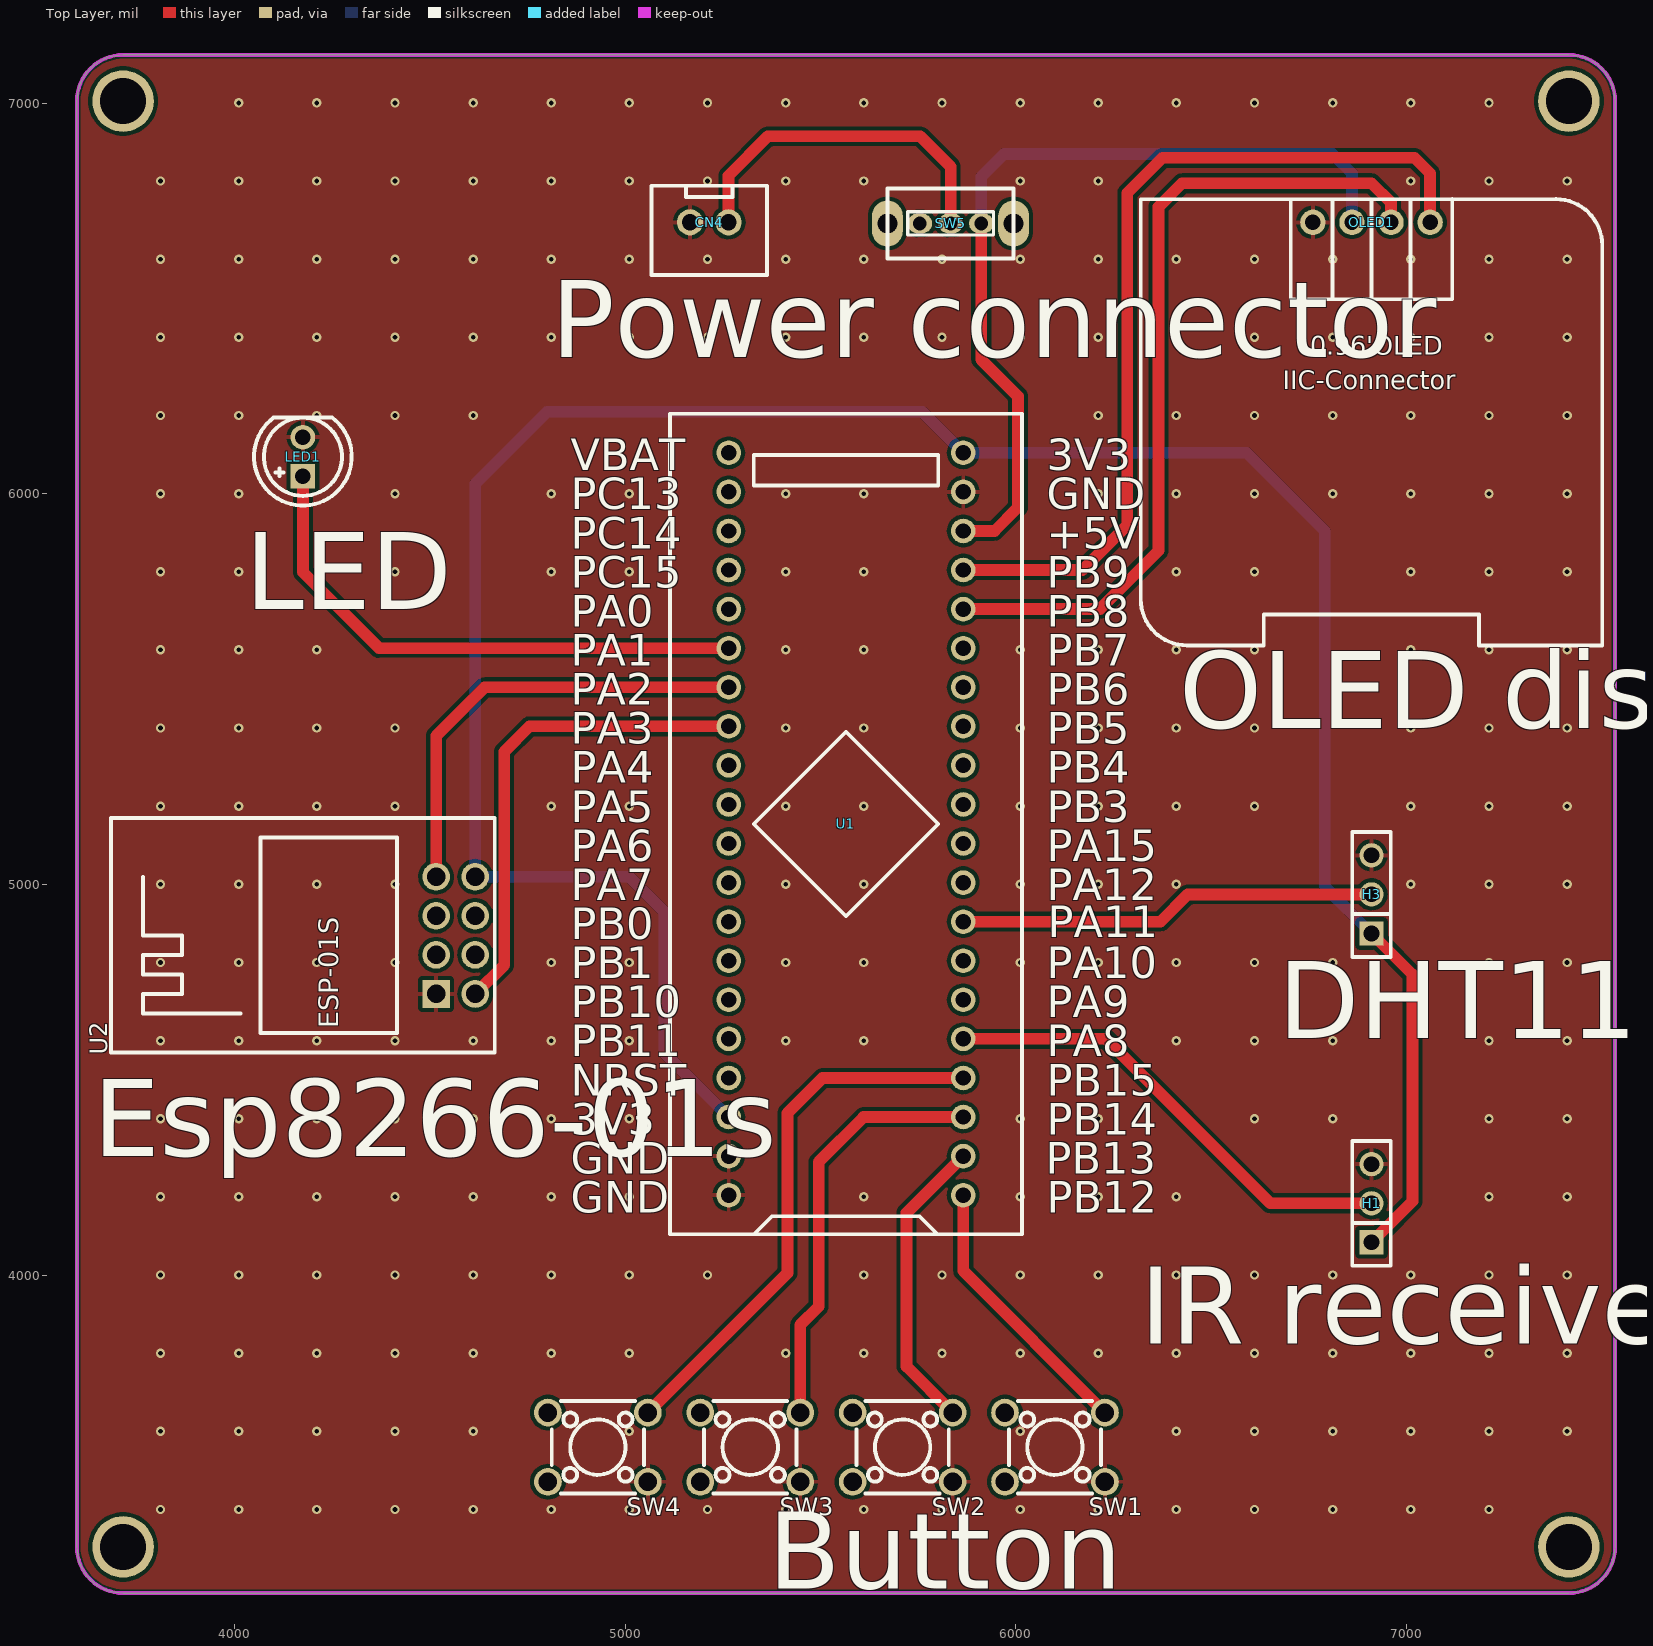
[diagram p0: Top Layer view]
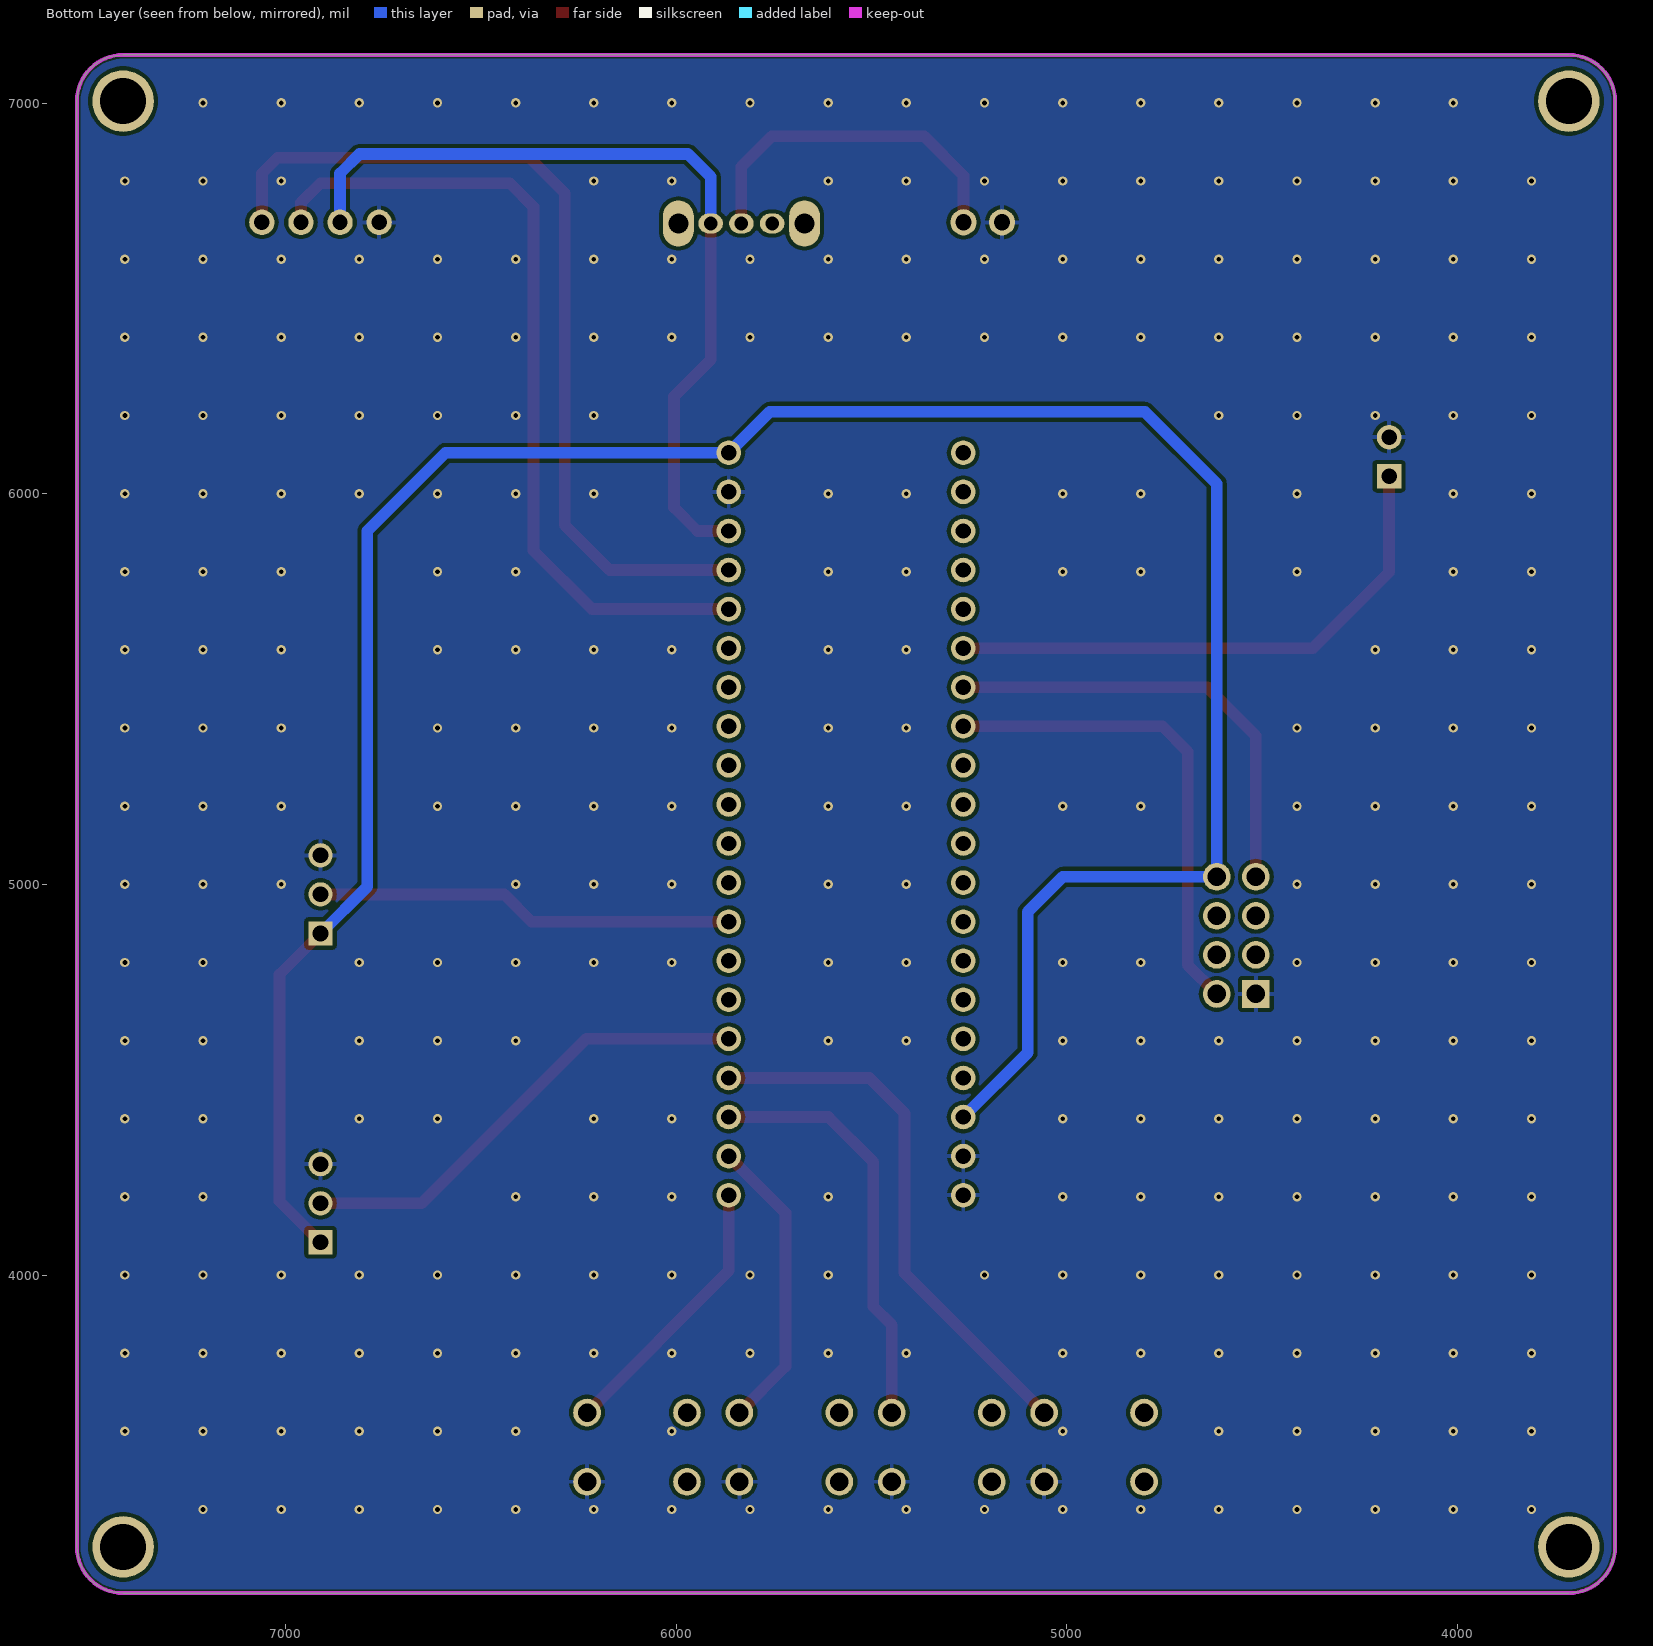
[diagram p1: Bottom Layer view, seen from below]
# Altium PCB MISC49868.pcbdoc
Units mil, origin at the board's own origin, x right, y up, seen from the top; angles counter-clockwise.
Board outline 3937.01 x 3937.01 mil, 2 copper layers (Top Layer, Bottom Layer), stack 62.206 mil thick; 12 components, 38 nets, 87 pads, 282 vias.

## Layer stack, top to bottom
Top Solder Mask Layer: solder mask 0.394, Dk 3.3
Top Layer: signal copper 1.379
Dielectric1: surface 59.449, FR4, Dk 4.5
Bottom Layer: signal copper 1.378
Bottom Solder Mask Layer: solder mask 0.394, Dk 3.3

## Board outline
3714.61,7123.5 ccw(c3714.61,7005.39) 3596.5,7005.39 3596.5,3304.61 ccw(c3714.61,3304.61) 3714.61,3186.5 7415.39,3186.5 ccw(c7415.39,3304.61) 7533.5,3304.61 7533.5,7005.39 ccw(c7415.39,7005.39) 7415.39,7123.5 3714.61,7123.5

## Design rules (kind name [scope] priority, off if disabled: settings)
BoardOutlineClearance copperThickness2oz_1 [All] p2 off: genericclearance=7.99 ignorepadtopadclearanceinfootprint=FALSE except(0: Arc-SplitContinuation Track-SplitContinuation SMDPad-SplitContinuation THPad-SplitContinuation Via-SplitContinuation Fill-SplitContinuation Region-SplitContinuation Poly-SplitContinuation Text-SplitContinuation Hole-SplitContinuation; 5.98: Arc-CutoutEdge Track-CutoutEdge SMDPad-CutoutEdge THPad-CutoutEdge Via-CutoutEdge Text-CutoutEdge; 6.9: Hole-OutlineEdge Hole-CutoutEdge; 10: Poly-OutlineEdge Poly-CutoutEdge; 11.81: Arc-OutlineEdge Track-OutlineEdge SMDPad-OutlineEdge THPad-OutlineEdge Via-OutlineEdge Fill-OutlineEdge Region-OutlineEdge Text-OutlineEdge Fill-CutoutEdge Region-CutoutEdge)
BoardOutlineClearance Plane_innerPlane_1 [All] p4 off: genericclearance=4.02 ignorepadtopadclearanceinfootprint=FALSE except(0: Arc-SplitContinuation Track-SplitContinuation SMDPad-SplitContinuation THPad-SplitContinuation Via-SplitContinuation Fill-SplitContinuation Region-SplitContinuation Poly-SplitContinuation Text-SplitContinuation Hole-SplitContinuation; 5.98: Arc-CutoutEdge Track-CutoutEdge SMDPad-CutoutEdge THPad-CutoutEdge Via-CutoutEdge Text-CutoutEdge; 6.9: Hole-OutlineEdge Hole-CutoutEdge; 10: Poly-OutlineEdge Poly-CutoutEdge; 11.81: Arc-OutlineEdge Track-OutlineEdge SMDPad-OutlineEdge THPad-OutlineEdge Via-OutlineEdge Fill-OutlineEdge Region-OutlineEdge Text-OutlineEdge Fill-CutoutEdge Region-CutoutEdge)
BoardOutlineClearance Copper_copperRegion_1 [All] p6 off: genericclearance=4.02 ignorepadtopadclearanceinfootprint=FALSE except(0: Arc-SplitContinuation Track-SplitContinuation SMDPad-SplitContinuation THPad-SplitContinuation Via-SplitContinuation Fill-SplitContinuation Region-SplitContinuation Poly-SplitContinuation Text-SplitContinuation Hole-SplitContinuation; 5.98: Arc-CutoutEdge Track-CutoutEdge SMDPad-CutoutEdge THPad-CutoutEdge Via-CutoutEdge Text-CutoutEdge; 6.9: Hole-OutlineEdge Hole-CutoutEdge; 10: Poly-OutlineEdge Poly-CutoutEdge; 11.81: Arc-OutlineEdge Track-OutlineEdge SMDPad-OutlineEdge THPad-OutlineEdge Via-OutlineEdge Fill-OutlineEdge Region-OutlineEdge Text-OutlineEdge Fill-CutoutEdge Region-CutoutEdge)
BoardOutlineClearance Copper_copperRegion_copperThickness1oz_1 [All] p8 off: genericclearance=4.02 ignorepadtopadclearanceinfootprint=FALSE except(0: Arc-SplitContinuation Track-SplitContinuation SMDPad-SplitContinuation THPad-SplitContinuation Via-SplitContinuation Fill-SplitContinuation Region-SplitContinuation Poly-SplitContinuation Text-SplitContinuation Hole-SplitContinuation; 5.98: Arc-CutoutEdge Track-CutoutEdge SMDPad-CutoutEdge THPad-CutoutEdge Via-CutoutEdge Text-CutoutEdge; 6.9: Hole-OutlineEdge Hole-CutoutEdge; 10: Poly-OutlineEdge Poly-CutoutEdge; 11.81: Arc-OutlineEdge Track-OutlineEdge SMDPad-OutlineEdge THPad-OutlineEdge Via-OutlineEdge Fill-OutlineEdge Region-OutlineEdge Text-OutlineEdge Fill-CutoutEdge Region-CutoutEdge)
BoardOutlineClearance Copper_copperRegion_Copper_copperRegion_1 [All] p10 off: genericclearance=4.02 ignorepadtopadclearanceinfootprint=FALSE except(0: Arc-SplitContinuation Track-SplitContinuation SMDPad-SplitContinuation THPad-SplitContinuation Via-SplitContinuation Fill-SplitContinuation Region-SplitContinuation Poly-SplitContinuation Text-SplitContinuation Hole-SplitContinuation; 5.98: Arc-CutoutEdge Track-CutoutEdge SMDPad-CutoutEdge THPad-CutoutEdge Via-CutoutEdge Text-CutoutEdge; 6.9: Hole-OutlineEdge Hole-CutoutEdge; 10: Poly-OutlineEdge Poly-CutoutEdge; 11.81: Arc-OutlineEdge Track-OutlineEdge SMDPad-OutlineEdge THPad-OutlineEdge Via-OutlineEdge Fill-OutlineEdge Region-OutlineEdge Text-OutlineEdge Fill-CutoutEdge Region-CutoutEdge)
BoardOutlineClearance copperThickness1oz_1 [All] p12: genericclearance=4.02 ignorepadtopadclearanceinfootprint=FALSE except(0: Arc-SplitContinuation Track-SplitContinuation SMDPad-SplitContinuation THPad-SplitContinuation Via-SplitContinuation Fill-SplitContinuation Region-SplitContinuation Poly-SplitContinuation Text-SplitContinuation Hole-SplitContinuation; 5.98: Arc-CutoutEdge Track-CutoutEdge SMDPad-CutoutEdge THPad-CutoutEdge Via-CutoutEdge Text-CutoutEdge; 6.9: Hole-OutlineEdge Hole-CutoutEdge; 10: Poly-OutlineEdge Poly-CutoutEdge; 11.81: Arc-OutlineEdge Track-OutlineEdge SMDPad-OutlineEdge THPad-OutlineEdge Via-OutlineEdge Fill-OutlineEdge Region-OutlineEdge Text-OutlineEdge Fill-CutoutEdge Region-CutoutEdge)
Clearance copperThickness2oz [All] p1 off: gap=7.99 ignorepadtopadclearanceinfootprint=FALSE except(5.98: SMDPad-Track SMDPad-SMDPad THPad-Track SMDPad-THPad THPad-THPad Track-Via SMDPad-Via THPad-Via Via-Via Fill-SMDPad Region-SMDPad Fill-THPad Region-THPad Fill-Via Region-Via Fill-Fill Fill-Region Region-Region Arc-Track Arc-SMDPad Arc-THPad Arc-Via Fill-Arc Region-Arc Arc-Arc Text-Track SMDPad-Text Text-THPad Text-Via Fill-Text Region-Text Arc-Text Text-Text; 6.9: Hole-Track Hole-SMDPad Hole-THPad Hole-Via Fill-Hole Region-Hole Hole-Arc Hole-Text; 10: Poly-Track Poly-SMDPad Poly-THPad Poly-Via Poly-Fill Poly-Region Poly-Poly Poly-Arc Poly-Text Poly-Hole; 11.81: Fill-Track Region-Track)
Clearance Plane_innerPlane [All] p3 off: gap=4.02 ignorepadtopadclearanceinfootprint=FALSE except(5.98: SMDPad-Track SMDPad-SMDPad THPad-Track SMDPad-THPad THPad-THPad Track-Via SMDPad-Via THPad-Via Via-Via Fill-SMDPad Region-SMDPad Fill-THPad Region-THPad Fill-Via Region-Via Fill-Fill Fill-Region Region-Region Arc-Track Arc-SMDPad Arc-THPad Arc-Via Fill-Arc Region-Arc Arc-Arc Text-Track SMDPad-Text Text-THPad Text-Via Fill-Text Region-Text Arc-Text Text-Text; 6.9: Hole-Track Hole-SMDPad Hole-THPad Hole-Via Fill-Hole Region-Hole Hole-Arc Hole-Text; 10: Poly-Track Poly-SMDPad Poly-THPad Poly-Via Poly-Fill Poly-Region Poly-Poly Poly-Arc Poly-Text Poly-Hole; 11.81: Fill-Track Region-Track)
Clearance Copper_copperRegion [All] p5 off: gap=4.02 ignorepadtopadclearanceinfootprint=FALSE except(5.98: SMDPad-Track SMDPad-SMDPad THPad-Track SMDPad-THPad THPad-THPad Track-Via SMDPad-Via THPad-Via Via-Via Fill-SMDPad Region-SMDPad Fill-THPad Region-THPad Fill-Via Region-Via Fill-Fill Fill-Region Region-Region Arc-Track Arc-SMDPad Arc-THPad Arc-Via Fill-Arc Region-Arc Arc-Arc Text-Track SMDPad-Text Text-THPad Text-Via Fill-Text Region-Text Arc-Text Text-Text; 6.9: Hole-Track Hole-SMDPad Hole-THPad Hole-Via Fill-Hole Region-Hole Hole-Arc Hole-Text; 10: Poly-Track Poly-SMDPad Poly-THPad Poly-Via Poly-Fill Poly-Region Poly-Poly Poly-Arc Poly-Text Poly-Hole; 11.81: Fill-Track Region-Track)
Clearance Copper_copperRegion_copperThickness1oz [All] p7 off: gap=4.02 ignorepadtopadclearanceinfootprint=FALSE except(5.98: SMDPad-Track SMDPad-SMDPad THPad-Track SMDPad-THPad THPad-THPad Track-Via SMDPad-Via THPad-Via Via-Via Fill-SMDPad Region-SMDPad Fill-THPad Region-THPad Fill-Via Region-Via Fill-Fill Fill-Region Region-Region Arc-Track Arc-SMDPad Arc-THPad Arc-Via Fill-Arc Region-Arc Arc-Arc Text-Track SMDPad-Text Text-THPad Text-Via Fill-Text Region-Text Arc-Text Text-Text; 6.9: Hole-Track Hole-SMDPad Hole-THPad Hole-Via Fill-Hole Region-Hole Hole-Arc Hole-Text; 10: Poly-Track Poly-SMDPad Poly-THPad Poly-Via Poly-Fill Poly-Region Poly-Poly Poly-Arc Poly-Text Poly-Hole; 11.81: Fill-Track Region-Track)
Clearance Copper_copperRegion_Copper_copperRegion [All] p9 off: gap=4.02 ignorepadtopadclearanceinfootprint=FALSE except(5.98: SMDPad-Track SMDPad-SMDPad THPad-Track SMDPad-THPad THPad-THPad Track-Via SMDPad-Via THPad-Via Via-Via Fill-SMDPad Region-SMDPad Fill-THPad Region-THPad Fill-Via Region-Via Fill-Fill Fill-Region Region-Region Arc-Track Arc-SMDPad Arc-THPad Arc-Via Fill-Arc Region-Arc Arc-Arc Text-Track SMDPad-Text Text-THPad Text-Via Fill-Text Region-Text Arc-Text Text-Text; 6.9: Hole-Track Hole-SMDPad Hole-THPad Hole-Via Fill-Hole Region-Hole Hole-Arc Hole-Text; 10: Poly-Track Poly-SMDPad Poly-THPad Poly-Via Poly-Fill Poly-Region Poly-Poly Poly-Arc Poly-Text Poly-Hole; 11.81: Fill-Track Region-Track)
Clearance copperThickness1oz [All] p11: gap=4.02 ignorepadtopadclearanceinfootprint=FALSE except(5.98: SMDPad-Track SMDPad-SMDPad THPad-Track SMDPad-THPad THPad-THPad Track-Via SMDPad-Via THPad-Via Via-Via Fill-SMDPad Region-SMDPad Fill-THPad Region-THPad Fill-Via Region-Via Fill-Fill Fill-Region Region-Region Arc-Track Arc-SMDPad Arc-THPad Arc-Via Fill-Arc Region-Arc Arc-Arc Text-Track SMDPad-Text Text-THPad Text-Via Fill-Text Region-Text Arc-Text Text-Text; 6.9: Hole-Track Hole-SMDPad Hole-THPad Hole-Via Fill-Hole Region-Hole Hole-Arc Hole-Text; 10: Poly-Track Poly-SMDPad Poly-THPad Poly-Via Poly-Fill Poly-Region Poly-Poly Poly-Arc Poly-Text Poly-Hole; 11.81: Fill-Track Region-Track)
DiffPairsRouting differentialPair [All] p1: maxlimit=6 minlimit=6 mostfreqgap=6 toplayer_minwidth=5 toplayer_prefwidth=10 toplayer_maxwidth=100 toplayer_mingap=6 toplayer_prefgap=6 toplayer_maxgap=6 bottomlayer_minwidth=5 bottomlayer_prefwidth=10 bottomlayer_maxwidth=100 bottomlayer_mingap=6 bottomlayer_prefgap=6 bottomlayer_maxgap=6 maxuncoupledlength=10
HoleToHoleClearance otherClearance [All] p1: gap=11.81 allowstackedmicrovias=TRUE
Length netLength [All] p1: minlimit=0 maxlimit=0
PasteMaskExpansion pasteMaskExpansion [All] p1: expansion=0
PlaneConnect innerPlane [All] p1: planeconnectstyle=Relief reliefexpansion=20 reliefentries=4 reliefconductorwidth=10 reliefairgap=10
PolygonConnect copperRegion_copperThickness1oz [All] p1 off: connectstyle=Relief reliefconductorwidth=10 reliefentries=4 polygonreliefangle="90 Angle" airgapwidth=10 via.connectstyle=Relief via.reliefconductorwidth=10 via.reliefentries=4 via.polygonreliefangle="90 Angle" via.airgapwidth=10
PolygonConnect copperRegion_Copper_copperRegion [All] p2 off: connectstyle=Relief reliefconductorwidth=10 reliefentries=4 polygonreliefangle="90 Angle" airgapwidth=10 via.connectstyle=Relief via.reliefconductorwidth=10 via.reliefentries=4 via.polygonreliefangle="90 Angle" via.airgapwidth=10
PolygonConnect copperRegion [All] p3: connectstyle=Relief reliefconductorwidth=10 reliefentries=4 polygonreliefangle="90 Angle" airgapwidth=10 via.connectstyle=Relief via.reliefconductorwidth=10 via.reliefentries=4 via.polygonreliefangle="90 Angle" via.airgapwidth=10
RoutingVias viaSize [All] p1: holewidth=12.01 width=24.02 viastyle="Through Hole" minholewidth=11.81 minwidth=19.68 maxholewidth=248.03 maxwidth=393.7
SolderMaskExpansion solderMaskExpansion [IsVia] p1: expansion=-1000 istentingtop=TRUE
SolderMaskExpansion solderMaskExpansion [All] p2: expansion=2 istentingtop=FALSE
Width copperThickness2oz_2 [All] p1 off: maxlimit=100 minlimit=8 preferedwidth=10
Width copperThickness1oz_2 [All] p2: maxlimit=100 minlimit=5 preferedwidth=10

## Components (designator, comment, footprint, x,y, rotation, side; value= is the part's Value field where it differs from the comment)
CN4 "XH2.54*2P_THT" CONN-TH_2P-P2.50-XH2.54-2P 5215,6695 r0 top
H1 "" HDR-TH_3P-P2.54-V-F 6910,4184.29 r90 top
H3 "" HDR-TH_3P-P2.54-V-F 6910,4974.81 r90 top
LED1 "" LED-TH_5mm 4175,6095 r90 top
OLED1 "" 0.96OLED_4P 6910,6695 r0 top
SW1 "" SW-TH_4P-L6.0-W6.0-P4.50-LS6.5 6099.85,3560 r180 top
SW2 "" SW-TH_4P-L6.0-W6.0-P4.50-LS6.5 5709.9,3560 r180 top
SW3 "" SW-TH_4P-L6.0-W6.0-P4.50-LS6.5 5319.95,3560 r180 top
SW4 "" SW-TH_4P-L6.0-W6.0-P4.50-LS6.5 4930,3560 r180 top
SW5 "" 拨动开关 5837.9,6692.05 r180 top
U1 "STM32F103C8T6-Card" CONN-TH_L53.3-W22.9_STM32F103C8T6-CARD 5565,5155 r90 top
U2 "ESP-01S" WIFIM-TH_ESP-01S 4566,4870 r90 top

## Footprints (in the part's own frame and the unit in brackets; to place one, negate y for a bottom-side part, rotate by r counter-clockwise, add the part's x,y. Pads: shape width x height; smd on the part's side, far side on the other; paste and mask are expansions set on the pad)
0.96OLED_4P [mm]
  round 1.65 hole 1 copper offset 0,0: 1(-3.81,-0.001) 2(-1.27,0.002) 3(1.27,0.002) 4(3.81,0.002)
  silkscreen extent -15,-27.5 15,1.5
CONN-TH_2P-P2.50-XH2.54-2P [mm]
  round 1.7 hole 1.05 paste+0 mask+0.05: 1(1.25,0) 2(-1.25,0)
  silkscreen extent -3.75,-3.42 3.75,2.37
CONN-TH_L53.3-W22.9_STM32F103C8T6-CARD [mm]
  round 1.6 hole 1: 1(-24.13,-7.62) 2(-21.59,-7.62) 3(-19.05,-7.62) 4(-16.51,-7.62) 5(-13.97,-7.62) 6(-11.43,-7.62) 7(-8.89,-7.62) 8(-6.35,-7.62) 9(-3.81,-7.62) 10(-1.27,-7.62) 11(1.27,-7.62) 12(3.81,-7.62) 13(6.35,-7.62) 14(8.89,-7.62) 15(11.43,-7.62) 16(13.97,-7.62) 17(16.51,-7.62) 18(19.05,-7.62) 19(21.59,-7.62) 20(24.13,-7.62) 21(24.13,7.62) 22(21.59,7.62) 23(19.05,7.62) 24(16.51,7.62) 25(13.97,7.62) 26(11.43,7.62) 27(8.89,7.62) 28(6.35,7.62) 29(3.81,7.62) 30(1.27,7.62) 31(-1.27,7.62) 32(-3.81,7.62) 33(-6.35,7.62) 34(-8.89,7.62) 35(-11.43,7.62) 36(-13.97,7.62) 37(-16.51,7.62) 38(-19.05,7.62) 39(-21.59,7.62) 40(-24.13,7.62)
  silkscreen extent -26.67,-11.43 26.67,11.43
HDR-TH_3P-P2.54-V-F [mil]
  rect 62x62 hole 40.16: 1(-100,0)
  round 62 hole 40.16: 2(0,0) 3(100,0)
  silkscreen extent -160,-49 160,49
LED-TH_5mm [mm]
  rect 1.6x1.6 hole 1 paste+0 mask+0.051: 1(-1.27,0)
  round 1.6 hole 1 paste+0 mask+0.051: 2(1.27,0)
  silkscreen extent -3.17,-3.17 2.54,3.17
SW-TH_4P-L6.0-W6.0-P4.50-LS6.5 [mm]
  round 1.8 hole 1.2: 1(-3.25,2.25) 2(3.25,2.25) 3(-3.25,-2.25) 4(3.25,-2.25)
  silkscreen extent -3,-3 3,3
WIFIM-TH_ESP-01S [mm]
  rect 1.8x1.8 hole 1.2: 1(-3.81,1.27)
  round 1.8 hole 1.2: 2(-1.27,1.27) 3(1.27,1.27) 4(3.81,1.27) 5(3.81,-1.27) 6(1.27,-1.27) 7(-1.27,-1.27) 8(-3.81,-1.27)
  silkscreen extent -7.62,-2.54 7.62,22.4
拨动开关 [mil]
  oval 63x51.2 hole 35.4 paste+0 mask+2: 1(-73.4,0) 2(5,0) 3(84,0)
  oval 78.7x118.1 hole 51.2 paste+0 mask+2: 4(166.7,0) 5(-156.1,0)
  silkscreen extent -156,-90 167,90

## Free pads (board coordinates)
  round 157.48 hole 118.11: 1(3714.61,7005.39) 1(3714.61,3304.61) 1(7415.39,7005.39) 1(7415.39,3304.61)

## Via types
v1: diameter 24.02, hole 12, Top Layer to Bottom Layer, 282 vias

## Nets (pads, with @x,y where several pads share a name; then routed paths per layer and width w, separated by ;. In a path a pad name is that pad's centre, name@x,y a point inside that pad or via, vN(x,y) a via of type N, cw(c..) or ccw(c..) an arc to the next point about the centre after c; other vN are vias at no path point)
$1N17118: CN4.1 SW5.2 | length 907
  Top Layer w30: CN4.1 5264.22,6814.22 5365,6915 5755,6915 5832.9,6837.1 SW5.2
+5V: OLED1.2 SW5.1 U1.18 | length 2168.6
  Top Layer w30: U1.18 5945,5905 6005,5965 6005,6250 5911.3,6343.7 SW5.1
  Bottom Layer w30: SW5.1 5911.3,6811.3 5970,6870 6810,6870 6860,6820 OLED1.2@6860,6695.05
GND: CN4.2 H1.3 H3.3 LED1.2 OLED1.1 SW1.1 SW2.1 SW3.1 SW4.1 U1.19 U1.39 U1.40 U2.1
  other v1: 3810.6,3400.6 4010.6,3400.6 4210.6,3400.6 4410.6,3400.6 4610.6,3400.6 4810.6,3400.6 5010.6,3400.6 5210.6,3400.6 5410.6,3400.6 5610.6,3400.6 5810.6,3400.6 6010.6,3400.6 6210.6,3400.6 6410.6,3400.6 6610.6,3400.6 6810.6,3400.6 7010.6,3400.6 7210.6,3400.6 3810.6,3600.6 4010.6,3600.6 4210.6,3600.6 4410.6,3600.6 4610.6,3600.6 5010.6,3600.6 6010.6,3600.6 6410.6,3600.6 6610.6,3600.6 6810.6,3600.6 7010.6,3600.6 7210.6,3600.6 7410.6,3600.6 3810.6,3800.6 4010.6,3800.6 4210.6,3800.6 4410.6,3800.6 4610.6,3800.6 4810.6,3800.6 5010.6,3800.6 5410.6,3800.6 5610.6,3800.6 5810.6,3800.6 6010.6,3800.6 6210.6,3800.6 6410.6,3800.6 6610.6,3800.6 6810.6,3800.6 7010.6,3800.6 7210.6,3800.6 7410.6,3800.6 3810.6,4000.6 4010.6,4000.6 4210.6,4000.6 4410.6,4000.6 4610.6,4000.6 4810.6,4000.6 5010.6,4000.6 5210.6,4000.6 5610.6,4000.6 5810.6,4000.6 6010.6,4000.6 6210.6,4000.6 6410.6,4000.6 6610.6,4000.6 6810.6,4000.6 7010.6,4000.6 7210.6,4000.6 7410.6,4000.6 3810.6,4200.6 4010.6,4200.6 4210.6,4200.6 4410.6,4200.6 4610.6,4200.6 4810.6,4200.6 5010.6,4200.6 5610.6,4200.6 6010.6,4200.6 6210.6,4200.6 6410.6,4200.6 7210.6,4200.6 7410.6,4200.6 3810.6,4400.6 4010.6,4400.6 4210.6,4400.6 4410.6,4400.6 4610.6,4400.6 4810.6,4400.6 5010.6,4400.6 6010.6,4400.6 6210.6,4400.6 6610.6,4400.6 6810.6,4400.6 7210.6,4400.6 7410.6,4400.6 3810.6,4600.6 4010.6,4600.6 4210.6,4600.6 4410.6,4600.6 4610.6,4600.6 4810.6,4600.6 5010.6,4600.6 5410.6,4600.6 5610.6,4600.6 6410.6,4600.6 6610.6,4600.6 6810.6,4600.6 7210.6,4600.6 7410.6,4600.6 3810.6,4800.6 4010.6,4800.6 4210.6,4800.6 4410.6,4800.6 4810.6,4800.6 5010.6,4800.6 5410.6,4800.6 5610.6,4800.6 6010.6,4800.6 6210.6,4800.6 6410.6,4800.6 6610.6,4800.6 6810.6,4800.6 7210.6,4800.6 7410.6,4800.6 3810.6,5000.6 4010.6,5000.6 4210.6,5000.6 4410.6,5000.6 5410.6,5000.6 5610.6,5000.6 6010.6,5000.6 6210.6,5000.6 6410.6,5000.6 7010.6,5000.6 7210.6,5000.6 7410.6,5000.6 3810.6,5200.6 4010.6,5200.6 4210.6,5200.6 4410.6,5200.6 4810.6,5200.6 5010.6,5200.6 5410.6,5200.6 5610.6,5200.6 6010.6,5200.6 6210.6,5200.6 6410.6,5200.6 6610.6,5200.6 7010.6,5200.6 7210.6,5200.6 7410.6,5200.6 3810.6,5400.6 4010.6,5400.6 4210.6,5400.6 4410.6,5400.6 5410.6,5400.6 5610.6,5400.6 6010.6,5400.6 6210.6,5400.6 6410.6,5400.6 6610.6,5400.6 7010.6,5400.6 7210.6,5400.6 7410.6,5400.6 3810.6,5600.6 4010.6,5600.6 4210.6,5600.6 5410.6,5600.6 5610.6,5600.6 6010.6,5600.6 6210.6,5600.6 6410.6,5600.6 6610.6,5600.6 7010.6,5600.6 7210.6,5600.6 7410.6,5600.6 3810.6,5800.6 4010.6,5800.6 4410.6,5800.6 4810.6,5800.6 5010.6,5800.6 5410.6,5800.6 5610.6,5800.6 6410.6,5800.6 6610.6,5800.6 7010.6,5800.6 7210.6,5800.6 7410.6,5800.6 3810.6,6000.6 4010.6,6000.6 4410.6,6000.6 4810.6,6000.6 5010.6,6000.6 5410.6,6000.6 5610.6,6000.6 6210.6,6000.6 6410.6,6000.6 6610.6,6000.6 6810.6,6000.6 7010.6,6000.6 7210.6,6000.6 7410.6,6000.6 3810.6,6200.6 4010.6,6200.6 4210.6,6200.6 4410.6,6200.6 4610.6,6200.6 6210.6,6200.6 6410.6,6200.6 6610.6,6200.6 6810.6,6200.6 7010.6,6200.6 7210.6,6200.6 7410.6,6200.6 3810.6,6400.6 4010.6,6400.6 4210.6,6400.6 4410.6,6400.6 4610.6,6400.6 4810.6,6400.6 5010.6,6400.6 5210.6,6400.6 5410.6,6400.6 5610.6,6400.6 5810.6,6400.6 6010.6,6400.6 6210.6,6400.6 6410.6,6400.6 6610.6,6400.6 6810.6,6400.6 7010.6,6400.6 7210.6,6400.6 7410.6,6400.6 3810.6,6600.6 4010.6,6600.6 4210.6,6600.6 4410.6,6600.6 4610.6,6600.6 4810.6,6600.6 5010.6,6600.6 5210.6,6600.6 5410.6,6600.6 5610.6,6600.6 5810.6,6600.6 6010.6,6600.6 6210.6,6600.6 6410.6,6600.6 6610.6,6600.6 6810.6,6600.6 7010.6,6600.6 7210.6,6600.6 7410.6,6600.6 3810.6,6800.6 4010.6,6800.6 4210.6,6800.6 4410.6,6800.6 4610.6,6800.6 4810.6,6800.6 5010.6,6800.6 5210.6,6800.6 5410.6,6800.6 5610.6,6800.6 6010.6,6800.6 6210.6,6800.6 7010.6,6800.6 7210.6,6800.6 7410.6,6800.6 4010.6,7000.6 4210.6,7000.6 4410.6,7000.6 4610.6,7000.6 4810.6,7000.6 5010.6,7000.6 5210.6,7000.6 5410.6,7000.6 5610.6,7000.6 5810.6,7000.6 6010.6,7000.6 6210.6,7000.6 6410.6,7000.6 6610.6,7000.6 6810.6,7000.6 7010.6,7000.6 7210.6,7000.6
NRST: U1.37
PA0: U1.25
PA1: LED1.1 U1.26 | length 1415.8
  Top Layer w30: LED1.1 4175,5800 4370,5605 U1.26
PA2: U1.27 U2.4 | length 1161.4
  Top Layer w30: U2.4 4516,5381 4640,5505 U1.27
PA3: U1.28 U2.8 | length 1252.6
  Top Layer w30: U2.8 4690,4794 4690,5340 4755,5405 U1.28
PA4: U1.29
PA5: U1.30
PA6: U1.31
PA7: U1.32
PA8: H1.2 U1.5 | length 1219.3
  Top Layer w30: U1.5 6230,4605 6650.71,4184.29 H1.2
PA9: U1.6
PA10: U1.7
PA11: H3.2 U1.8 | length 1073.9
  Top Layer w30: U1.8 6370,4905 6439.81,4974.81 H3.2
PA12: U1.9
PA15: U1.10
PB0: U1.33
PB1: U1.34
PB3: U1.11
PB4: U1.12
PB5: U1.13
PB6: U1.14
PB7: U1.15
PB8: OLED1.3 U1.16 | length 2132.6
  Top Layer w30: U1.16 6215,5705 6365,5855 6365,6735 6425,6795 6910,6795 6960,6745 OLED1.3@6960,6695.05
PB9: OLED1.4 U1.17 | length 2271.4
  Top Layer w30: U1.17 6170,5805 6285,5920 6285,6770 6375,6860 7020,6860 7060,6820 OLED1.4@7060,6695.05
PB10: U1.35
PB11: U1.36
PB12: SW1.3 U1.1 | length 706.7
  Top Layer w30: U1.1 5865,4011.38 SW1.3
PB13: SW2.3 U1.2 | length 765.3
  Top Layer w30: SW2.3@5837.85,3648.58 5720,3766.43 5720,4160 U1.2
PB14: SW3.3 U1.3 | length 1078.6
  Top Layer w30: SW3.3 5447.9,3872.9 5495,3920 5495,4290 5610,4405 U1.3
PB15: SW4.3 U1.4 | length 1401.6
  Top Layer w30: SW4.3 5415,4005.63 5415,4415 5505,4505 U1.4
PC13: U1.22
PC14: U1.23
PC15: U1.24
VBAT: U1.21
VCC: H1.1 H3.1 U1.20 U1.38 U2.5 | length 6454.6
  Top Layer w30: H1.1 7015,4189.3 7015,4769.81 H3.1
  Bottom Layer w30: U1.38 5100,4570 5100,4930 5010,5020 U2.5 4616,6026 4800,6210 5760,6210 U1.20 6590,6105 6790,5905 6790,4994.81 H3.1
pads on no net: SW1.2 SW1.4 SW2.2 SW2.4 SW3.2 SW3.4 SW4.2 SW4.4 SW5.3 SW5.4 SW5.5 U2.2 U2.3 U2.6 U2.7

## Polygon pours and split planes (outlines as drawn)
GND on Bottom Layer (solid, remove dead copper, pour order 2): 3525,7245 3525,3080 7700,3080 7700,7245
GND on Top Layer (solid, remove dead copper, pour order 2): 3000,7415 3000,3000 7930,3000 7930,7415

## Keep-outs
Board Outline Layer:
  the board outline again, w10

## Silkscreen, mask and mechanical layers (free items; w line width, h text height)
Top Silkscreen Layer:
  text "Power connector" at 4810,6350 h196.85
  text "VBAT" at 4860.95,6060 h80
  text "3V3" at 6079.16,6060 h80
  text "PC13" at 4860.95,5960 h80
  text "GND" at 6079.16,5960 h80
  text "PC14" at 4860.95,5860 h80
  text "+5V" at 6079.16,5860 h80
  text "PC15" at 4860.95,5760 h80
  text "PB9" at 6079.16,5760 h80
  text "LED" at 4027.96,5705 h196.85
  text "PA0" at 4860.95,5660 h80
  text "PB8" at 6079.16,5660 h80
  text "PA1" at 4860.95,5560 h80
  text "PB7" at 6079.16,5560 h80
  text "PA2" at 4860.95,5460 h80
  text "PB6" at 6079.16,5460 h80
  text "OLED display" at 6418.02,5400.08 h196.85
  text "PA3" at 4860.95,5360 h80
  text "PB5" at 6079.16,5360 h80
  text "PA4" at 4860.95,5260 h80
  text "PB4" at 6079.16,5260 h80
  text "PA5" at 4860.95,5160 h80
  text "PB3" at 6079.16,5160 h80
  text "PA6" at 4860.95,5060 h80
  text "PA15" at 6079.16,5060 h80
  text "PA7" at 4860.95,4960 h80
  text "PA12" at 6079.16,4960 h80
  text "PA11" at 6080.95,4865 h80
  text "PB0" at 4860.95,4860 h80
  text "PB1" at 4860.95,4760 h80
  text "PA10" at 6079.16,4760 h80
  text "PB10" at 4860.95,4660 h80
  text "PA9" at 6079.16,4660 h80
  text "DHT11" at 6671.39,4607.17 h196.85
  text "PB11" at 4860.95,4560 h80
  text "PA8" at 6079.16,4560 h80
  text "NRST" at 4860.95,4460 h80
  text "PB15" at 6079.16,4460 h80
  text "3V3" at 4860.95,4360 h80
  text "PB14" at 6079.16,4360 h80
  text "Esp8266-01s" at 3638.14,4305 h196.85
  text "GND" at 4860.95,4260 h80
  text "PB13" at 6075.95,4260 h80
  text "GND" at 4860.95,4160 h80
  text "PB12" at 6079.16,4160 h80
  text "IR receiver module" at 6318.74,3825 h196.85
  text "Button" at 5366.3,3198.15 h196.85